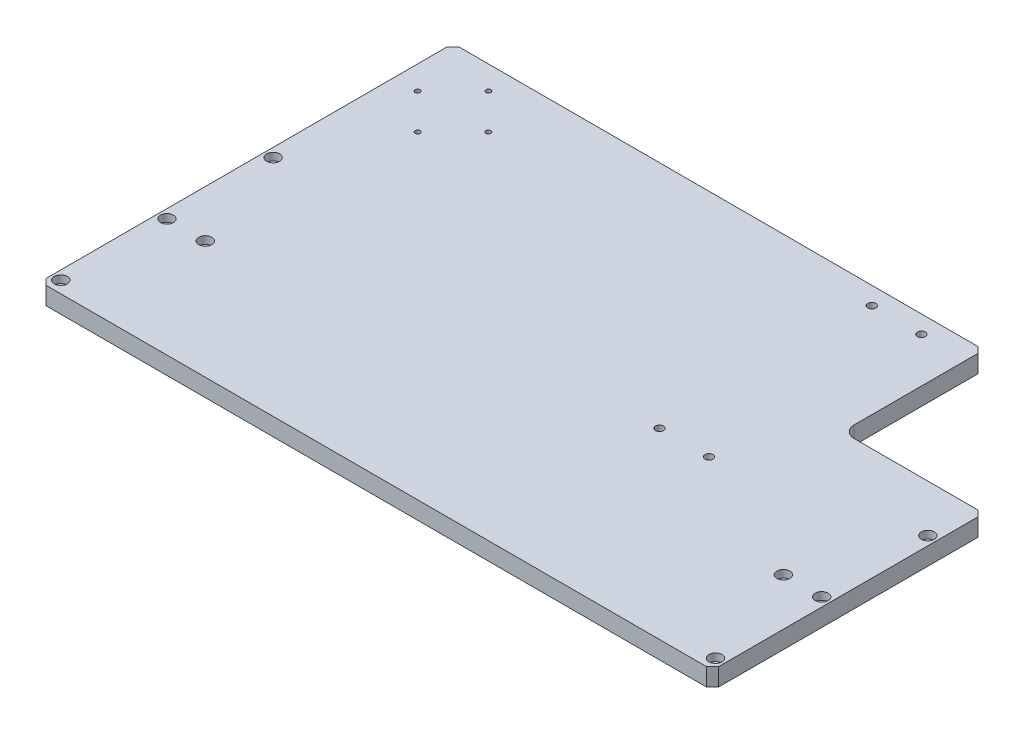
from build123d import *

# Parameters (mm, degrees)
SKETCH_1_W                   = 570
SKETCH_1_H                   = 350
EXTRUDE_1_DEPTH              = 7.5
CHAMFER_1_SIZE               = 5
HOLE_WIZARD_M5_1_D           = 4.2
HOLE_WIZARD_M8_1_D           = 6.8
HOLE_WIZARD_M6_1_D           = 6.6
HOLE_WIZARD_M6_1_DEPTH       = 17
HOLE_WIZARD_M6_1_CBORE_D     = 11
HOLE_WIZARD_M6_1_CBORE_DEPTH = 6.4
HOLE_WIZARD_M6_1_TIP         = 1.982840043
HOLE_WIZARD_M6_2_D           = 6.6
HOLE_WIZARD_M6_2_DEPTH       = 17
HOLE_WIZARD_M6_2_CBORE_D     = 11
HOLE_WIZARD_M6_2_CBORE_DEPTH = 6.4
HOLE_WIZARD_M6_2_TIP         = 1.982840043
SKETCH_10_W                  = 120
SKETCH_10_H                  = 120
CUT_EXTRUDE_1_DEPTH          = 335.776044543
FILLET_1_R                   = 10
CHAMFER_2_SIZE               = 5


with BuildPart() as part:
    # 草图1 → 凸台-拉伸1 (new, symmetric)
    with BuildSketch(Plane(origin=(0, 0, 0), x_dir=(1, 0, 0), z_dir=(0, 1, 0))):
        Rectangle(SKETCH_1_W, SKETCH_1_H)
    extrude(amount=EXTRUDE_1_DEPTH, both=True)

    # 倒角1
    chamfer_1_edges = [part.edges().sort_by_distance(p)[0] for p in [
        (-285, 0, -175),
        (285, 0, -175),
        (285, 0, 175),
        (-285, 0, 175),
    ]]
    chamfer(chamfer_1_edges, length=CHAMFER_1_SIZE)

    # M5 螺纹孔1 (through all)
    with Locations(Plane(origin=(0, 7.5, 0), x_dir=(1, 0, 0), z_dir=(0, 1, 0))):
        with Locations((-265, 125), (-235, 95), (-235, 155), (-205, 125)):
            Hole(HOLE_WIZARD_M5_1_D / 2)

    # M8 螺纹孔1 (through all)
    with Locations(Plane(origin=(0, 7.5, 0), x_dir=(1, 0, 0), z_dir=(0, 1, 0))):
        with Locations((85, -20), (127, -20), (127, 160), (85, 160)):
            Hole(HOLE_WIZARD_M8_1_D / 2)

    # M6 六角凹头螺钉的柱形沉头孔1
    with Locations(Plane(origin=(0, 7.5, 0), x_dir=(1, 0, 0), z_dir=(0, 1, 0))):
        with Locations((-277.5, 15), (-277.5, -165), (277.5, 15), (277.5, -165), (-277.5, -75), (277.5, -75)):
            CounterBoreHole(HOLE_WIZARD_M6_1_D / 2, HOLE_WIZARD_M6_1_CBORE_D / 2, HOLE_WIZARD_M6_1_CBORE_DEPTH, depth=HOLE_WIZARD_M6_1_DEPTH)
            with Locations((0, 0, -(HOLE_WIZARD_M6_1_DEPTH + HOLE_WIZARD_M6_1_TIP / 2))):  # 118° drill point
                Cone(0, HOLE_WIZARD_M6_1_D / 2, HOLE_WIZARD_M6_1_TIP, mode=Mode.SUBTRACT)

    # M6 六角凹头螺钉的柱形沉头孔2
    with Locations(Plane(origin=(0, 7.5, 0), x_dir=(1, 0, 0), z_dir=(0, 1, 0))):
        with Locations((-245, -75), (245, -75)):
            CounterBoreHole(HOLE_WIZARD_M6_2_D / 2, HOLE_WIZARD_M6_2_CBORE_D / 2, HOLE_WIZARD_M6_2_CBORE_DEPTH, depth=HOLE_WIZARD_M6_2_DEPTH)
            with Locations((0, 0, -(HOLE_WIZARD_M6_2_DEPTH + HOLE_WIZARD_M6_2_TIP / 2))):  # 118° drill point
                Cone(0, HOLE_WIZARD_M6_2_D / 2, HOLE_WIZARD_M6_2_TIP, mode=Mode.SUBTRACT)

    # 草图10 → 切除-拉伸1 (cut, through all)
    with BuildSketch(Plane(origin=(0, 7.5, 0), x_dir=(1, 0, 0), z_dir=(0, 1, 0))):
        with Locations((225, 115)):
            Rectangle(SKETCH_10_W, SKETCH_10_H)
    extrude(amount=-CUT_EXTRUDE_1_DEPTH, mode=Mode.SUBTRACT)

    # 圆角1
    fillet_1_edges = [part.edges().sort_by_distance(p)[0] for p in [
        (165, 0, -55),
    ]]
    fillet(fillet_1_edges, radius=FILLET_1_R)

    # 倒角2
    chamfer_2_edges = [part.edges().sort_by_distance(p)[0] for p in [
        (285, 0, -55),
        (165, 0, -175),
    ]]
    chamfer(chamfer_2_edges, length=CHAMFER_2_SIZE)


solid = part.part
